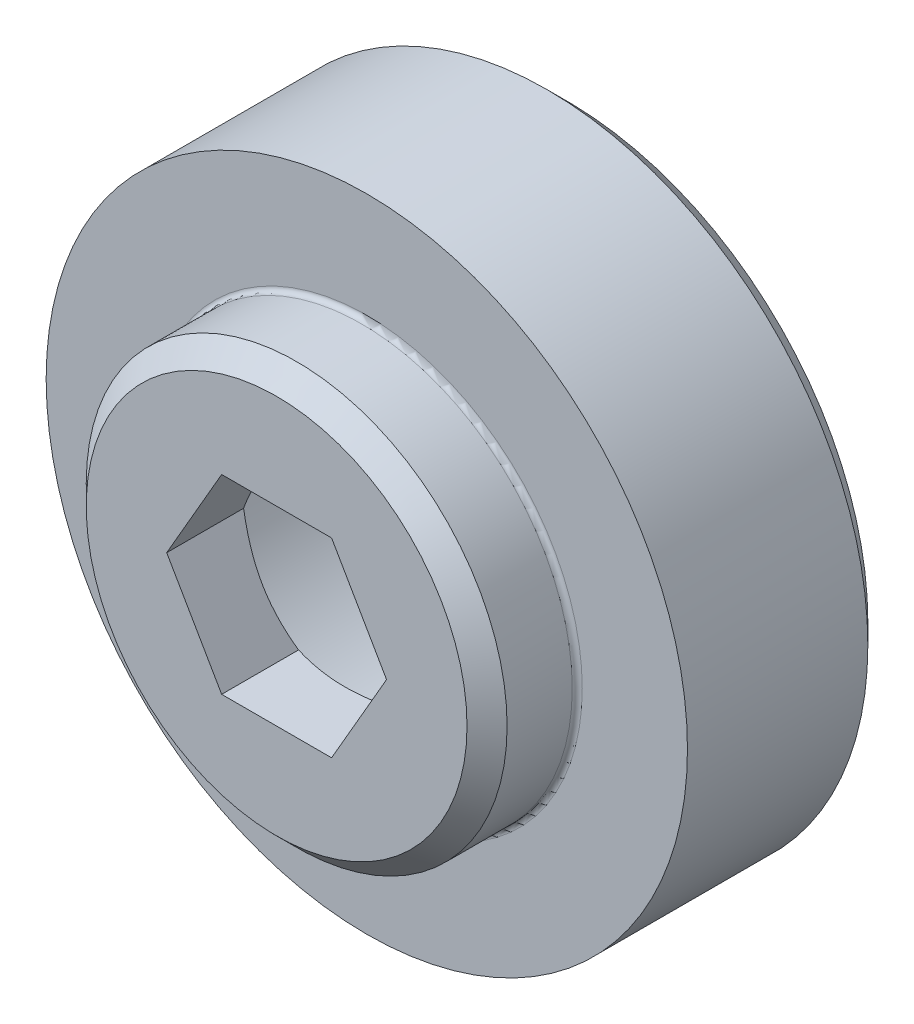
SolidWorks part; units mm, degrees
material "Q345 "
ref_plane "前视基准面" through (0, 0, 0) normal (0, 0, 1) x (1, 0, 0)
ref_plane "上视基准面" through (0, 0, 0) normal (0, 1, 0) x (1, 0, 0)
ref_plane "右视基准面" through (0, 0, 0) normal (1, 0, 0) x (0, 0, -1)
sketch "草图1" plane through (0, 0, 0) normal (0, 0, 1) x (1, 0, 0)
  circle A0 centre (0, 0) radius 32
  dimension "D1" = 64
extrude "凸台-拉伸1" add sketch "草图1" along normal blind 20
cosmetic thread "装饰螺纹线1" parameters "D1"=20, "D2"=57.505
sketch "草图2" plane through (0, 0, 20) normal (0, 0, 1) x (1, 0, 0)
  circle A0 centre (0, 0) radius 21
  dimension "D1" = 42
extrude "凸台-拉伸2" add sketch "草图2" along normal blind 9
hole_wizard "M48 螺纹孔1" positions "3D草图1" profile "草图4" tap size "M48" standard "GB"
sketch3d "3D草图1"
  circle A0 centre (0, 0, 0) radius 32 construction
  point P0 (0, 0, 0)
  point P5 (0, 0, 32)
sketch "草图4" plane through (0, 0, 0) normal (1, 0, 0) x (0, 1, 0)
  line L0 (0, 0) -> (0, 27.9185)
  line L1 (0, 27.9185) -> (21.5, 15)
  line L2 (21.5, 15) -> (21.5, 0)
  line L5 (21.5, 0) -> (0, 0)
  line L10 (0, 27.9185) -> (-21.5, 15) construction
  line L11 (0, -6.35) -> (0, 107.95) construction
  dimension "螺纹孔钻头直径" = 43
  dimension "螺纹孔钻头深度" = 15
  dimension "导头角度" = 118
cosmetic thread "孔螺蚊线2" parameters "D1"=10, "D2"=48
sketch "草图5" plane through (0, 0, 29) normal (0, 0, 1) x (1, 0, 0)
  line L0 (0, 0) -> (10.9697, 0) construction
  line L1 (10.9697, 0) -> (5.4848, 9.5)
  line L2 (5.4848, 9.5) -> (-5.4848, 9.5)
  line L3 (-5.4848, 9.5) -> (-10.9697, 0)
  line L4 (-10.9697, 0) -> (-5.4848, -9.5)
  line L5 (-5.4848, -9.5) -> (5.4848, -9.5)
  line L6 (5.4848, -9.5) -> (10.9697, 0)
  circle A0 centre (0, 0) radius 9.5 construction
  dimension "D1" = 19
extrude "切除-拉伸1" cut sketch "草图5" against normal through all
chamfer "倒角2" distance 2 angle 45 1 edges at (32, 0, 0)
chamfer "倒角3" distance 2 angle 45 1 edges at (21, 0, 29)
fillet "圆角1" radius 0.5 1 edges at (21, 0, 20)
